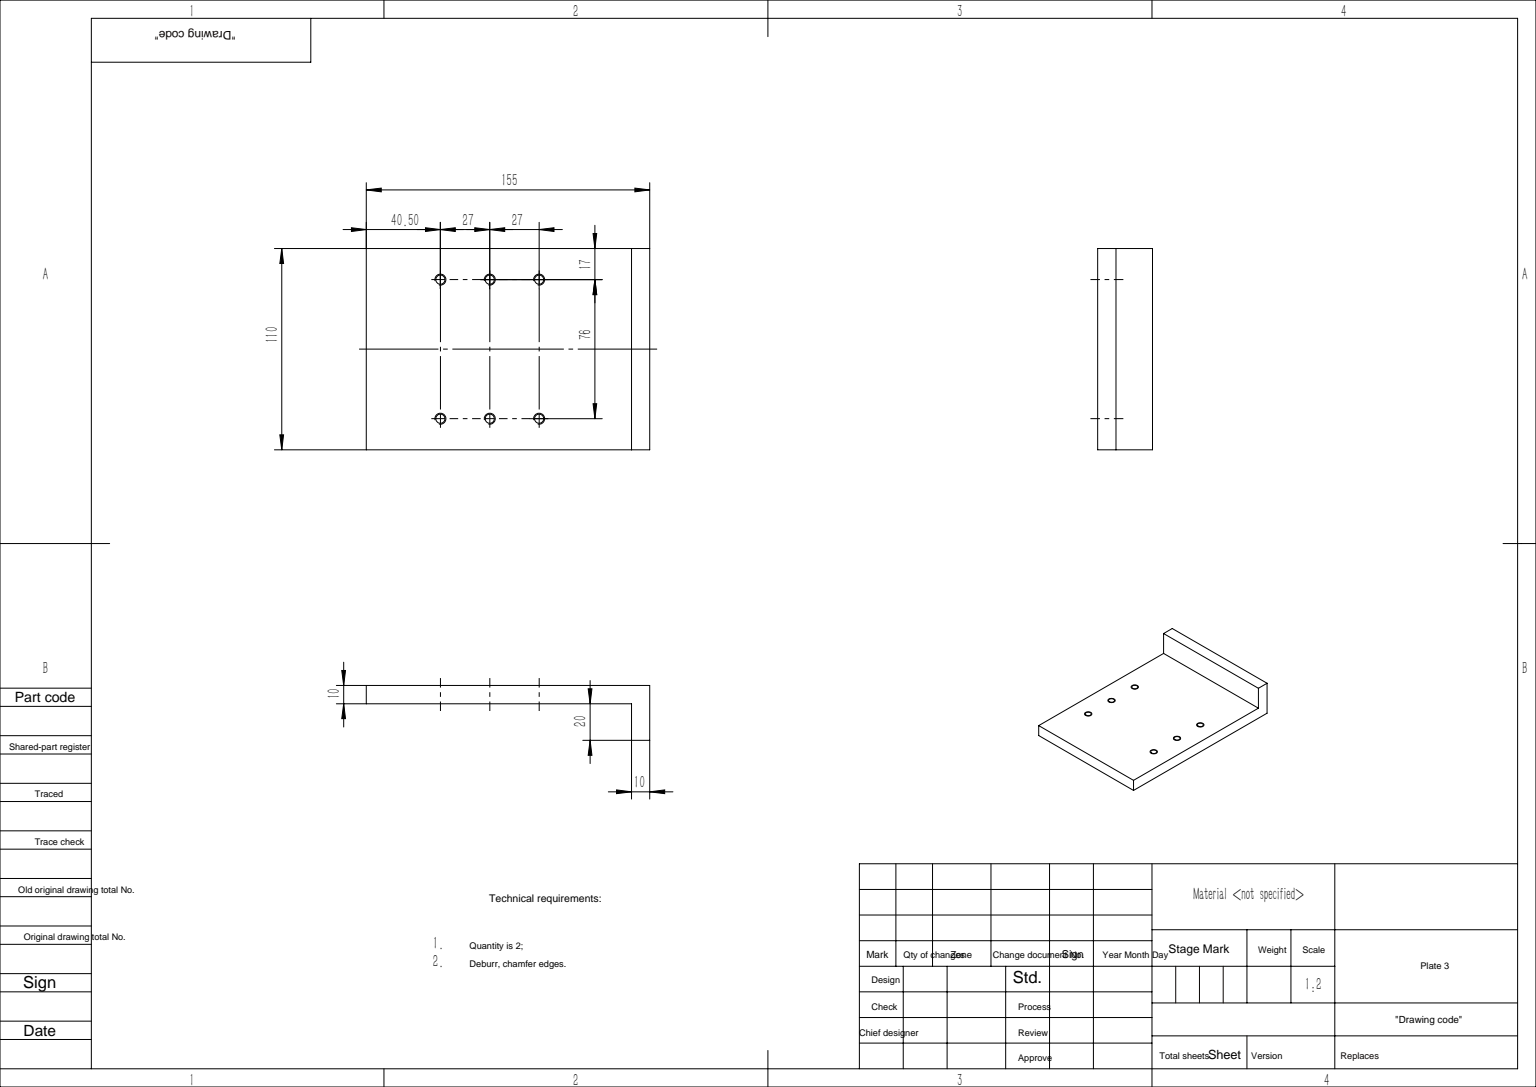
SolidWorks part; units mm, degrees
ref_plane "前视基准面" through (0, 0, 0) normal (0, 0, 1) x (1, 0, 0)
ref_plane "上视基准面" through (0, 0, 0) normal (0, 1, 0) x (1, 0, 0)
ref_plane "右视基准面" through (0, 0, 0) normal (1, 0, 0) x (0, 0, -1)
sketch "草图2" plane through (0, 0, 0) normal (0, 1, 0) x (1, 0, 0)
  line L1 (-55, -67.5) -> (55, -67.5)
  line L2 (-55, -67.5) -> (-55, 67.5)
  line L3 (-55, 67.5) -> (55, 67.5)
  line L4 (55, -67.5) -> (55, 67.5)
  line L5 (-55, -67.5) -> (55, 67.5) construction
  line L6 (-55, 67.5) -> (55, -67.5) construction
  point P0 (0, 0)
  dimension "D1" = 135
  dimension "D2" = 110
extrude "凸台-拉伸1" add sketch "草图2" along normal blind 10
hole_wizard "M6 螺纹孔1" positions "草图6" profile "草图5" tap size "M6" standard "GB" end condition through all
sketch "草图6" plane through (0, 10, 0) normal (0, 1, 0) x (1, 0, 0)
  point P0 (-38, 27)
  point P5 (-38, 0)
  point P8 (38, 0)
  point P11 (-38, -27)
  point P14 (38, -27)
  point P18 (38, 27)
sketch "草图5" plane through (-38, 10, -27) normal (1, 0, 0) x (0, 0, 1)
  line L0 (0, 0) -> (0, 10)
  line L1 (0, 10) -> (2.5, 10)
  line L2 (2.5, 10) -> (2.5, 0)
  line L5 (2.5, 0) -> (0, 0)
  line L11 (0, -6.35) -> (0, 107.95) construction
  dimension "通孔螺纹孔钻头直径" = 5
  dimension "通孔螺纹孔钻头深度" = 10
cosmetic thread "孔螺蚊线1" parameters "D2"=6
cosmetic thread "孔螺蚊线2" parameters "D2"=6
cosmetic thread "孔螺蚊线3" parameters "D2"=6
cosmetic thread "孔螺蚊线4" parameters "D2"=6
cosmetic thread "孔螺蚊线5" parameters "D2"=6
cosmetic thread "孔螺蚊线6" parameters "D2"=6
sketch "草图11" plane through (0, 0, 0) normal (0, -1, 0) x (1, 0, 0)
  line L0 (55, 67.5) -> (55, -67.5) construction
  line L1 (-55, -67.5) -> (55, -67.5)
  line L2 (-55, -67.5) -> (-55, -87.5)
  line L3 (-55, -87.5) -> (55, -87.5)
  line L4 (55, -67.5) -> (55, -87.5)
  dimension "D1" = 20
extrude "凸台-拉伸6" add sketch "草图11" against normal blind 10
sketch "草图15" plane through (0, 0, -87.5) normal (0, 0, -1) x (-1, 0, 0)
  line L0 (-55, 10) -> (-55, 0) construction
  line L1 (-55, 30) -> (55, 30)
  line L2 (-55, 30) -> (-55, 0)
  line L3 (-55, 0) -> (55, 0)
  line L4 (55, 30) -> (55, 0)
  line L6 (55, 10) -> (55, 0) construction
  dimension "D1" = 30
extrude "凸台-拉伸7" add sketch "草图15" against normal blind 10
